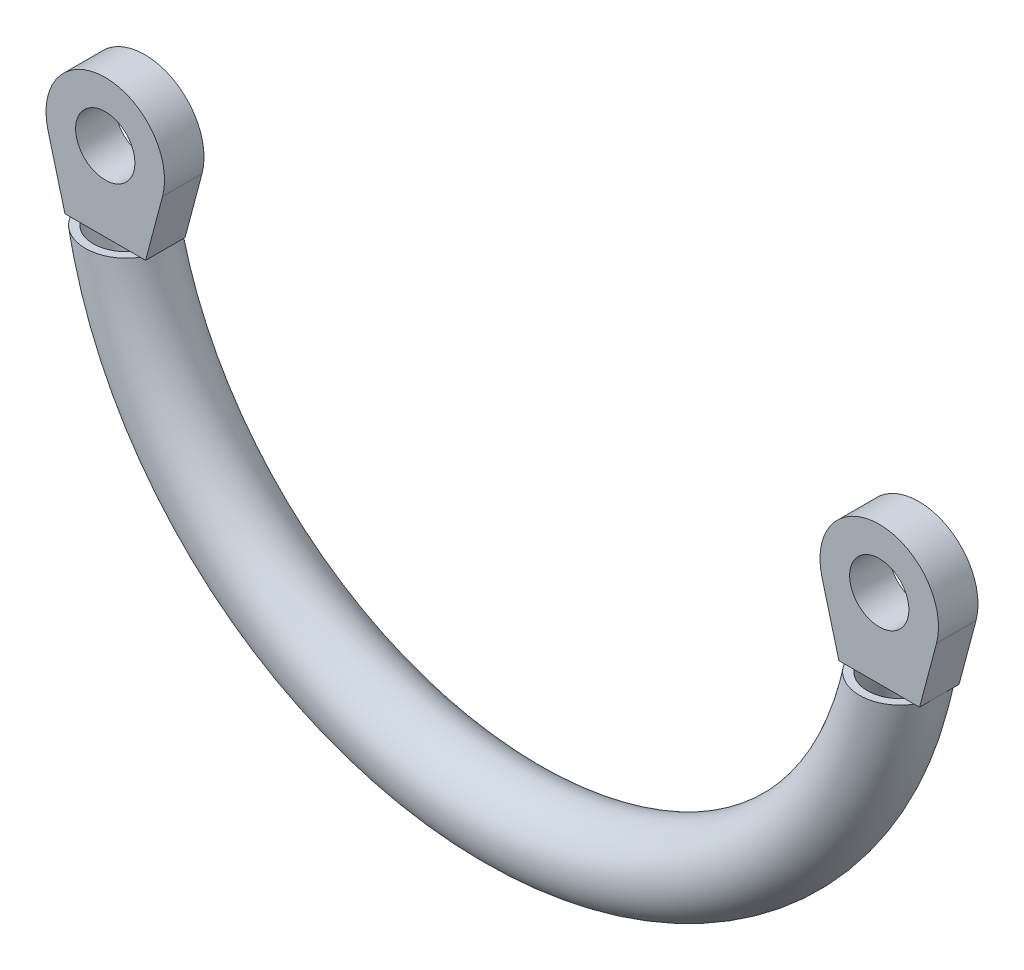
SolidWorks part; units mm, degrees
material "Q235-A"
ref_plane "前视基准面" through (0, 0, 0) normal (0, 0, 1) x (1, 0, 0)
ref_plane "上视基准面" through (0, 0, 0) normal (0, 1, 0) x (1, 0, 0)
ref_plane "右视基准面" through (0, 0, 0) normal (1, 0, 0) x (0, 0, -1)
sketch "草图1" plane through (0, 0, 0) normal (0, 0, 1) x (1, 0, 0)
  line L0 (0, 0) -> (0, -100) construction
  circle A0 centre (0, 0) radius 100
  dimension "D1" = 200
sketch "草图2" plane through (0, 0, 0) normal (1, 0, 0) x (0, 0, -1)
  line L0 (0, 100) -> (0, -100) construction
  line L1 (0, 0) -> (0, -100) construction
  circle A0 centre (0, -100) radius 10
  circle A1 centre (0, -100) radius 8
  dimension "D1" = 20
  dimension "D2" = 2
sweep "扫描1" add profiles "草图2" path "草图1"
sketch "草图3" plane through (0, 0, 0) normal (0, 0, 1) x (1, 0, 0)
  line L0 (-124.8211, -20) -> (0, -20)
  line L1 (0, -20) -> (127.8232, -20)
  line L2 (127.8232, -20) -> (127.8232, 142.661)
  line L3 (127.8232, 142.661) -> (-124.8211, 142.661)
  line L4 (-124.8211, 142.661) -> (-124.8211, -20)
  dimension "D1" = 20
extrude "切除-拉伸1" cut sketch "草图3" against normal through all both and the other way through all
sketch "草图4" plane through (0, 0, 0) normal (0, 0, 1) x (1, 0, 0)
  line L0 (-108.1665, -20) -> (-87.7496, -20) construction
  line L1 (-97.9581, -20) -> (-97.9581, 0) construction
  line L2 (-108.1665, -20) -> (-112.4555, -3.8502)
  line L3 (-87.7496, -20) -> (-83.4606, -3.8502)
  line L4 (-108.1665, -20) -> (-87.7496, -20)
  circle A0 centre (-97.9581, 0) radius 7.5
  arc A1 (-83.4606, -3.8502) -> (-112.4555, -3.8502) centre (-97.9581, 0) ccw
  arc A2 (-87.7496, -20) -> (87.7496, -20) centre (0, 0) ccw construction
  dimension "D1" = 15
  dimension "D2" = 30
  dimension "D3" = 20
extrude "凸台-拉伸1" add sketch "草图4" along normal mid plane 10
mirror "镜向1" about plane through (0, 0, 0) normal (1, 0, 0) of "凸台-拉伸1"
